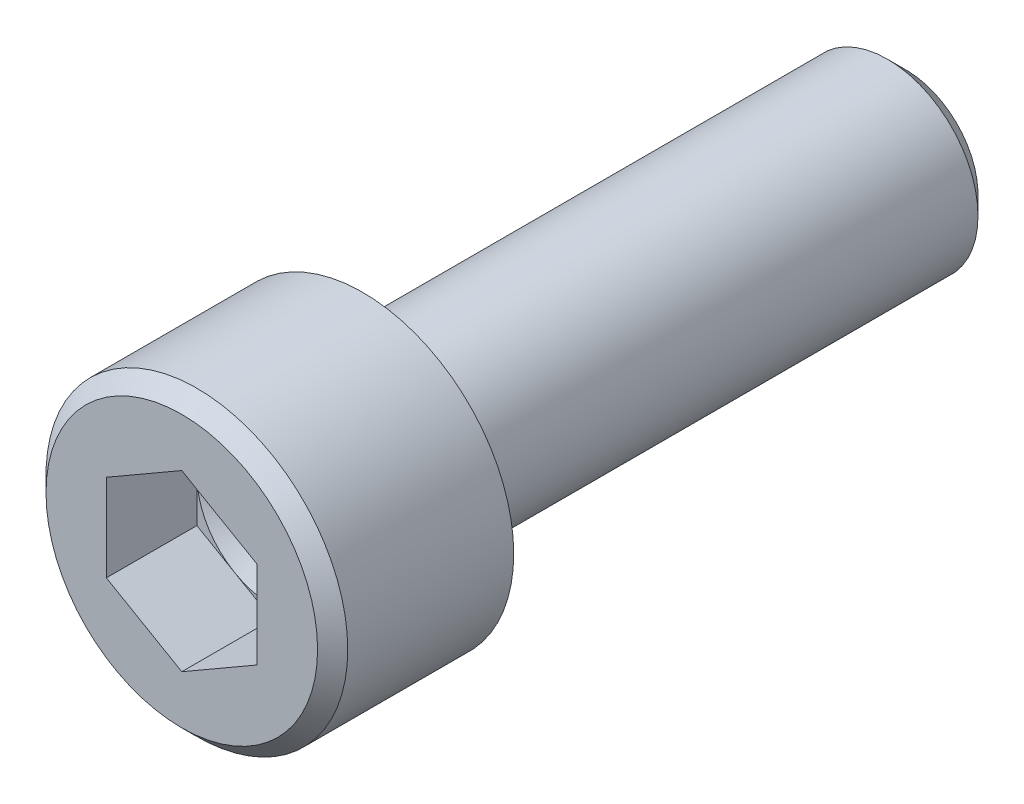
from build123d import *

# Parameters (mm, degrees)
SKETCH_1_W          = 5
SKETCH_1_H          = 6
SKETCH_2_R          = 3
EXTRUDE_1_DEPTH     = 18
CUT_EXTRUDE_1_DEPTH = 3
CHAMFER_1_SIZE      = 0.5
CHAMFER_2_SIZE      = 0.6135


with BuildPart() as part:
    # 草图1 → 旋转1 (revolve)
    with BuildSketch(Plane(origin=(0, 0, 0), x_dir=(1, 0, 0), z_dir=(0, 1, 0))):
        with Locations((2.5, -3)):
            Rectangle(SKETCH_1_W, SKETCH_1_H)
    revolve(axis=Axis((0, 0, 0), (0, 0, 1)))

    # 草图2 → 凸台-拉伸1 (add)
    with BuildSketch(Plane(origin=(0, 0, 0), x_dir=(-1, 0, 0), z_dir=(0, 0, -1))):
        Circle(SKETCH_2_R)
    extrude(amount=EXTRUDE_1_DEPTH)

    # 草图3 → 切除-拉伸1 (cut)
    with BuildSketch(Plane.XY.offset(6)):
        Polygon((2.5, 1.443375673), (0, 2.886751346), (-2.5, 1.443375673), (-2.5, -1.443375673), (0, -2.886751346), (2.5, -1.443375673), align=None)
    extrude(amount=-CUT_EXTRUDE_1_DEPTH, mode=Mode.SUBTRACT)

    # 草图4 → 切除-旋转1 (revolve, cut)
    with BuildSketch(Plane.XZ):
        Polygon((2.5, 3), (0, 3), (0, 1.556624327), align=None)
    revolve(axis=Axis((0, 0, 3), (0, 0, -1)), mode=Mode.SUBTRACT)

    # 倒角1
    chamfer_1_edges = [part.edges().sort_by_distance(p)[0] for p in [
        (-5, 0, 6),
    ]]
    chamfer(chamfer_1_edges, length=CHAMFER_1_SIZE)

    # 倒角2
    chamfer_2_edges = [part.edges().sort_by_distance(p)[0] for p in [
        (3, 0, -18),
    ]]
    chamfer(chamfer_2_edges, length=CHAMFER_2_SIZE)


solid = part.part
